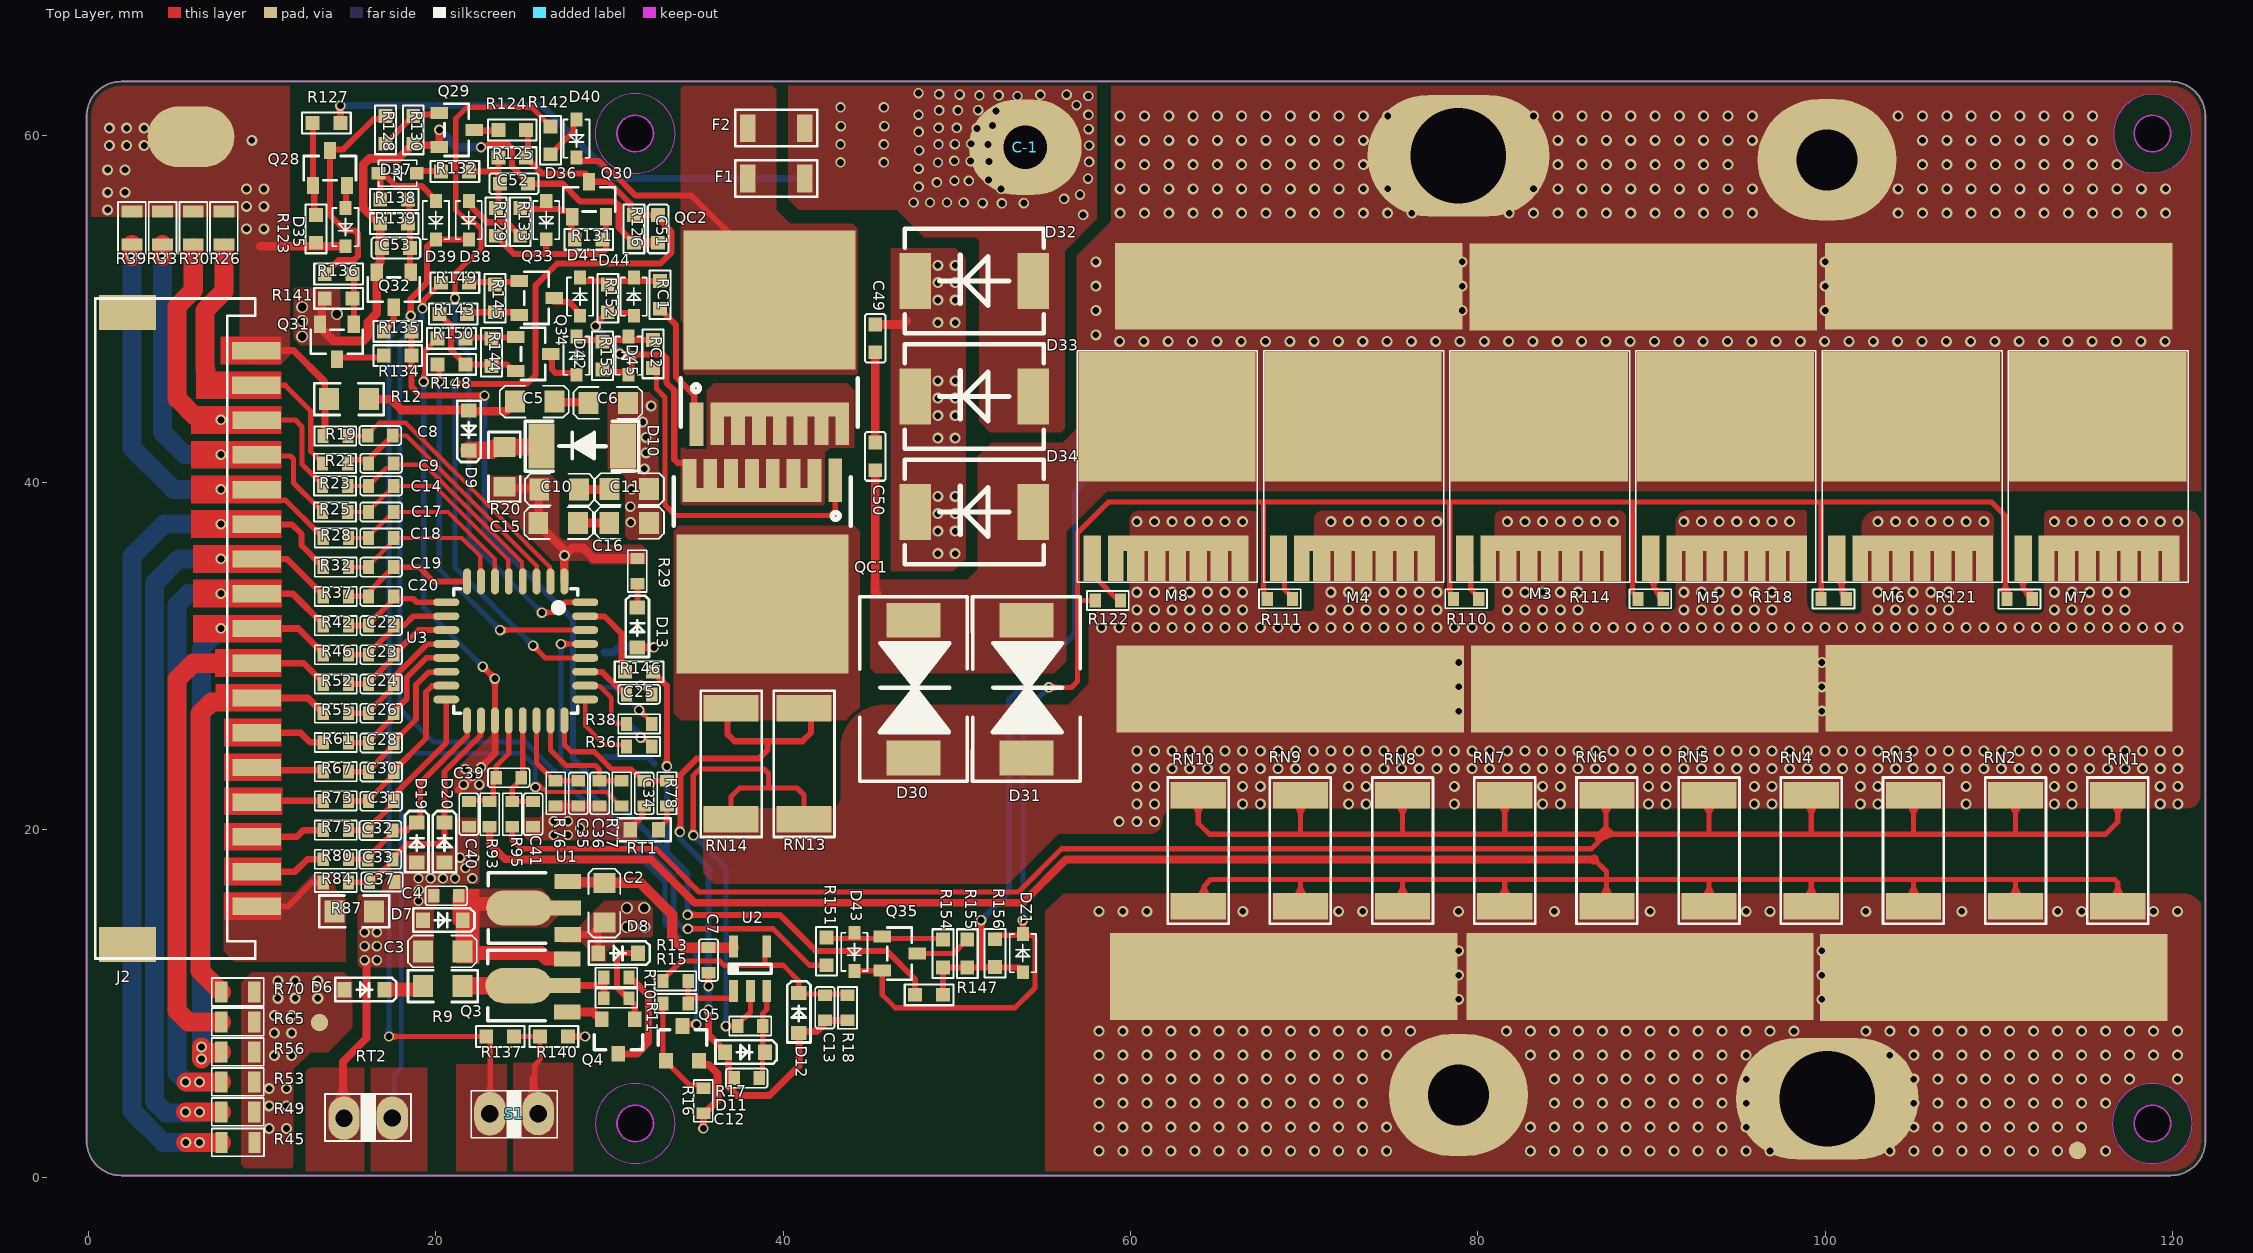
[diagram p0: Top Layer view]
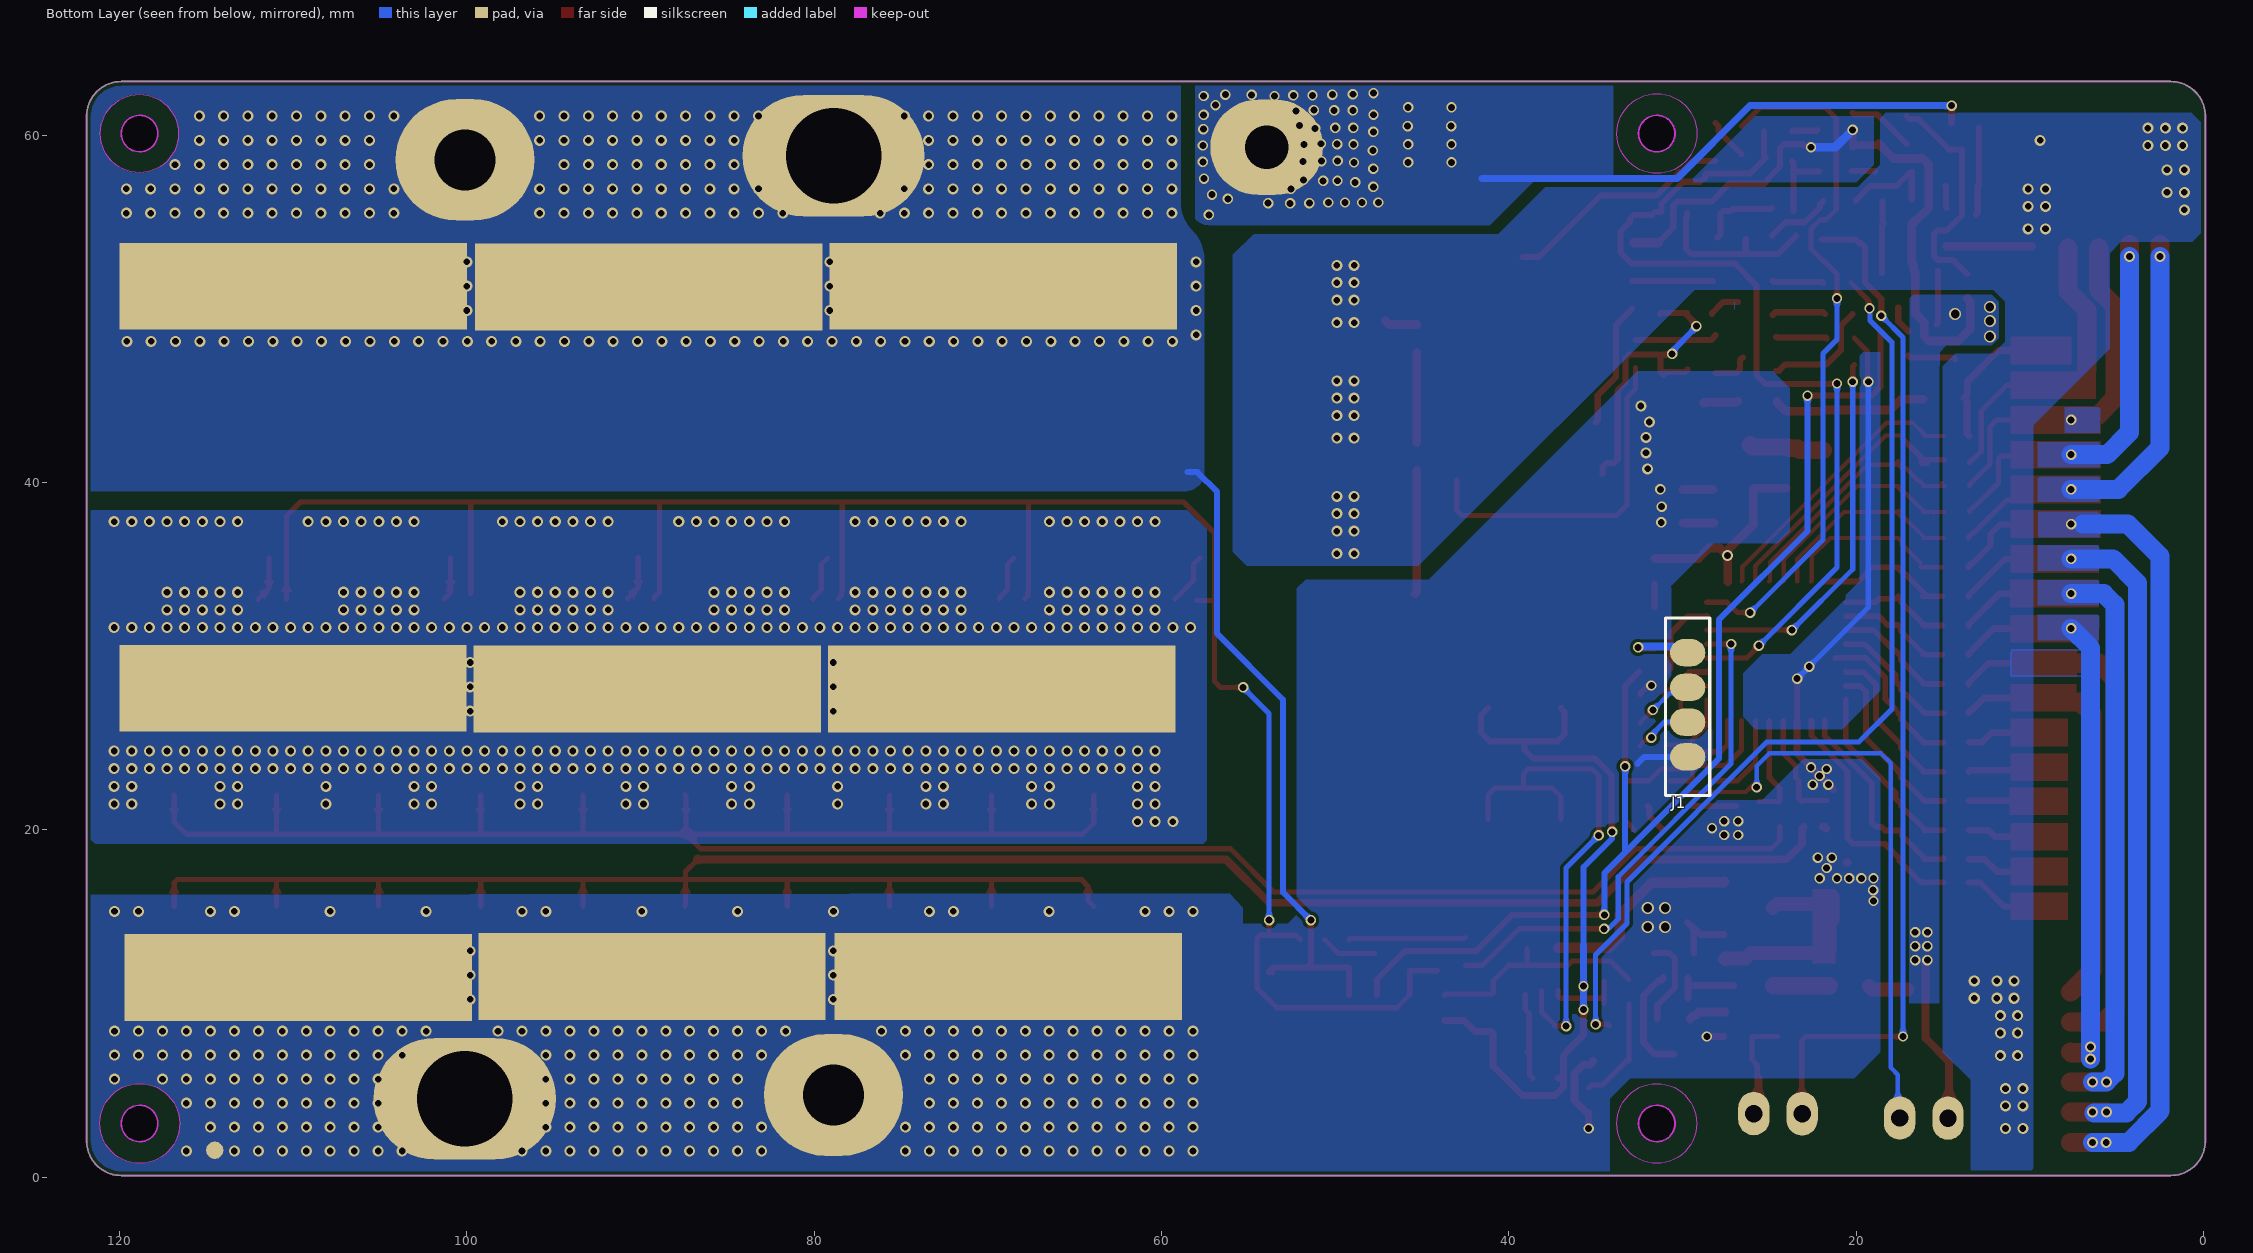
[diagram p1: Bottom Layer view, seen from below]
# Altium PCB MISC86327.PcbDoc (part 1 of 2)
Units mm, origin at the board's own origin, x right, y up, seen from the top; angles counter-clockwise.
Board outline 122 x 63 mm, 2 copper layers (Top Layer, Bottom Layer); 198 components, 117 nets, 551 pads, 998 vias.
Unrouted connection lines stored in the file: 65.

## Layer stack, top to bottom (the 12.6 mil dielectric is the usual default, probably not edited)
Top Solder: solder mask 0.0102, Solder Resist, Dk 3.5
Top Layer: signal copper 0.0356
Dielectric 1: dielectric 0.32, FR-4, Dk 4.8
Bottom Layer: signal copper 0.0356
Bottom Solder: solder mask 0.0102, Solder Resist, Dk 3.5

## Board outline
-0.11,2.09 -0.11,61.09 cw(c1.89,61.09) 1.89,63.09 119.89,63.09 cw(c119.89,61.09) 121.89,61.09 121.89,2.09 cw(c119.89,2.09) 119.89,0.09 1.89,0.09 cw(c1.89,2.09)
cut-out: 31.48,59.04 cw(c31.48,60.09) 30.43,60.09 cw(c31.48,60.09) 31.48,61.14 cw(c31.48,60.09) 32.53,60.09 cw(c31.48,60.09)
cut-out: 30.43,3.09 ccw(c31.48,3.09) 31.48,2.04 ccw(c31.48,3.09) 32.53,3.09 ccw(c31.48,3.09) 31.48,4.14 ccw(c31.48,3.09)
cut-out: 117.79,3.09 ccw(c118.84,3.09) 118.84,2.04 ccw(c118.84,3.09) 119.89,3.09 ccw(c118.84,3.09) 118.84,4.14 ccw(c118.84,3.09)
cut-out: 117.79,60.09 ccw(c118.84,60.09) 118.84,59.04 ccw(c118.84,60.09) 119.89,60.09 ccw(c118.84,60.09) 118.84,61.14 ccw(c118.84,60.09)

## Design rules (kind name [scope] priority, off if disabled: settings)
Clearance [All] p1: gap=0.2 ignorepadtopadclearanceinfootprint=FALSE except(0: Arc-Hole Track-Hole SMDPad-Hole THPad-Hole Via-Hole Fill-Hole Poly-Hole Region-Hole Text-Hole)
ComponentClearance [All] p1 off: gap=0.254 collisioncheckmode=3 verticalgap=0.254 showdistances=FALSE
Height [All] p1 off: minheight=0 maxheight=25.4 prefheight=12.7
HoleSize [All] p1: absolutevalues=TRUE maxlimit=10 minlimit=0.025 maxpercent=80.000 minpercent=20.000
HoleToHoleClearance [All] p1 off: gap=0 allowstackedmicrovias=TRUE
MinimumSolderMaskSliver [All] p1 off: minsoldermaskwidth=0
PolygonConnect [All] p1: connectstyle=Direct reliefconductorwidth=0.254 reliefentries=4 polygonreliefangle="90 Angle" airgapwidth=0.254
RoutingVias [All] p1: holewidth=0.5 width=0.8 viastyle="Through Hole" minholewidth=0.4 minwidth=0.6 maxholewidth=0.711 maxwidth=1.27
SilkToSilkClearance [All] p1 off: silktosilkclearance=0
SilkToSolderMaskClearance [IsPad] p1 off: minsilkscreentomaskgap=0 clearancetoexposedcopper=TRUE
SolderMaskExpansion [All] p1: expansion=0.102 istentingtop=FALSE
SupplyNets "Schematic Supply Nets_2" [InNet('DSGD1')] p1: voltage=0.000
SupplyNets "Schematic Supply Nets_5" [InNet('C-')] p2: voltage=0.000
SupplyNets "Schematic Supply Nets" [InNet('BC16')] p3: voltage=0.000
SupplyNets "Schematic Supply Nets_6" [InNet('GND1')] p4: voltage=0.000
SupplyNets "Schematic Supply Nets_4" [InNet('5V')] p5: voltage=0.000
SupplyNets "Schematic Supply Nets_3" [InNet('GND')] p6: voltage=0.000
Width [All] p1: maxlimit=20 minlimit=0.2 preferedwidth=0.3
23 further rules are at their usual default settings.

## Components (designator, comment, footprint, x,y, rotation, side; value= is the part's Value field where it differs from the comment)
C2 "10uF/25V" C0805 29.7,15.8 r270 top
C3 "2.2uF/50V" C0805 20.4,13 r180 top
C4 "0.1uF" C0603M 20.6,16.2 r180 top
C5 "2.2uF/100V" C0805 25.69,44.66 r180 top
C6 "2.2uF/100V" C0805 29.93,44.58 r180 top
C7 "10nF" C0603M 35.7,12.5 r270 top
C8 "0.1uF" C0603M 16.8,42.7 r0 top
C9 "0.1uF" C0603M 16.845,41.1 r0 top
C10 "0.1uF/100V" C0805 27.095,39.582 r0 top
C11 "0.1uF/100V" C0805 31.135,39.612 r0 top
C12 "0.47uF" C0603M 37.9,5.7 r180 top
C13 "0.47uF" C0603M 42.4,9.753 r270 top
C14 "0.1uF" C0603M 16.847,39.8 r0 top
C15 "2.2uF/100V" C0805 27.039,37.662 r0 top
C16 "2.2uF/100V" C0805 31.125,37.672 r0 top
C17 "0.1uF" C0603M 16.847,38.3 r0 top
C18 "0.1uF" C0603M 16.847,36.806 r0 top
C19 "0.1uF" C0603M 16.847,35.123 r0 top
C20 "0.1uF" C0603M 16.847,33.441 r0 top
C22 "0.1uF" C0603M 16.847,31.759 r0 top
C23 "0.1uF" C0603M 16.847,30.077 r0 top
C24 "0.1uF" C0603M 16.847,28.395 r0 top
C25 "1uF/25V" C0603M 31.7,27.8 r0 top
C26 "0.1uF" C0603M 16.847,26.713 r0 top
C28 "0.1uF" C0603M 16.847,25 r0 top
C30 "0.1uF" C0603M 16.847,23.33 r0 top
C31 "0.1uF" C0603M 16.847,21.648 r0 top
C32 "0.1uF" C0603M 16.8,19.966 r0 top
C33 "0.1uF" C0603M 16.8,18.3 r0 top
C34 "102" C0603M 32,22.1 r90 top
C35 "102" C0603M 28.2,22.1 r90 top
C36 "102" C0603M 29.43,22.1 r90 top
C37 "1uF" C0603M 16.9,17 r0 top
C39 "102" C0603M 24.2,23 r180 top
C40 "1uF" C0603M 21.9,20.9 r270 top
C41 "1uF" C0603M 25.6,20.9 r270 top
C49 "0.1uF" C0603A 45.3,48.3 r90 top
C50 "0.1uF" C0603A 45.3,41.5 r90 top
C51 "0.1uF" C0603A 32.8,54.6 r90 top
C52 "0.1uF" C0603A 24.5,57.2 r180 top
C53 "0.1uF" C0603A 17.7,53.5 r0 top
C-1 "Pth" 4*3 53.94,59.3 r0 top locked
D6 "1N4148WS" SOD-323-E 15.9,10.8 r0 top
D7 "15V" SOD-323-E 20.4,14.8 r0 top
D8 "15V" SOD-323-E 30.5,12.9 r0 top
D9 "BAV21WS" SOD-323-E 21.9,43 r270 top
D10 "SMAJ64A" SMA 28.43,42.09 r180 top
D11 "1N4148WS" SOD-323-E 37.8,7.2 r0 top
D12 "1N4148WS" SOD-323-E 40.9,9.453 r90 top
D13 "BAV21WS" SOD-323-E 31.6,31.65 r90 top
D19 "BAT46WS" SOD-323-E 18.9,19.261 r90 top
D20 "BAT46WS" SOD-323-E 20.5,19.261 r90 top
D30 "SMDJ150CA" SMC-BI 47.5,28.1 r90 top
D31 "SMDJ150CA" SMC-BI 54,28.1 r90 top
D32 "RS5M" SMC_MDO-214AB) 51,51.6 r180 top
D33 "RS5M" SMC_MDO-214AB) 51,44.95 r180 top
D34 "RS5M" SMC_MDO-214AB) 51,38.3 r180 top
D35 "15V" SOD323(A+K-) 14.8,54.7 r90 top
D36 "5.6V" SOD323(A+K-) 26.357,55.106 r90 top
D37 "1N4148WS" SOD323(A+K-) 17.8,57.8 r0 top
D38 "1N4148WS" SOD323(A+K-) 21.9,55.1 r90 top
D39 "1N4148WS" SOD323(A+K-) 20,55.1 r90 top
D40 "BAV21WS" SOD323(A+K-) 28.1,59.8 r90 top
D41 "1N4148WS" SOD323(A+K-) 28.3,50.7 r270 top
D42 "BAV21WS" SOD323(A+K-) 28.1,47.3 r270 top
D43 "BAV21WS" SOD323(A+K-) 44.1,12.975 r90 top
D44 "15V" SOD323(A+K-) 31.4,50.7 r270 top
D45 "15V" SOD323(A+K-) 31.1,47.3 r270 top
DZ1 "15V" SOD323(A+K-) 53.8,12.9 r270 top
F1 "5A/125VAC" R1206L 39.6,57.5 r0 top
F2 "40A/72V" R1206L 39.6,60.4 r0 top
J1 "UART_M" CON4/2.0 29.7,27.2 r270 bottom
J2 "PH-2.0mm-17P right-angle connector without latch" "HY2.0WT-17A/P 卧贴带扣耐温260℃" 5.965,31.59 r90 top locked
M3 "SP012N02AGHTO" TOLL#1 83.487,39.712 r0 top
M4 "SP012N02AGHTO" TOLL#1 72.768,39.712 r0 top
M5 "SP012N02AGHTO" TOLL#1 94.205,39.712 r0 top
M6 "SP012N02AGHTO" TOLL#1 104.923,39.712 r0 top
M7 "SP012N02AGHTO" TOLL#1 115.642,39.712 r0 top
M8 "SP012N02AGHTO" TOLL#1 62.05,39.712 r0 top
Q3 "DXT5551" SOT-89BCE 26.159,11.028 r90 top
Q4 "MMBT5551" SOT-23S 30.5,8.1 r180 top
Q5 "MMBT5551" SOT-23S 34.2,7.7 r0 top
Q28 "MMBT5401" SOT23-3_BEC 13.9,58.1 r0 top
Q29 "MMBT5551" SOT23-3_BEC 21.2,60.3 r270 top
Q30 "MMBT5401" SOT23-3_BEC 28.825,56.3 r0 top
Q31 "MMBT5551" SOT23-3_BEC 14.3,48.1 r180 top
Q32 "MMBT5551" SOT23-3_BEC 17.575,51.1 r180 top
Q33 "MMBT5401" SOT23-3_BEC 25.8,50.625 r270 top
Q34 "MMBT5401" SOT23-3_BEC 25.6,47.4 r270 top
Q35 "MMBT5401" SOT23-3_BEC 46.7,12.875 r270 top
QC1 "N MOS*" TOLL#2 38.8,36.5 r180 top
QC2 "N MOS*" TOLL#2 39.2,47 r0 top
R9 "200R" R0805 20.4,11 r180 top
R10 "100K" R0603m 30.4,11.5 r0 top
R11 "3M" R0603m 30.4,10.3 r0 top
R12 "1K" R0805 15,44.8 r0 top
R13 "470K 1%" R0603m 33.8,11.3 r0 top
R15 "100K 1%" R0603m 33.8,10 r180 top
R16 "1M" R0603m 35.4,4.4 r90 top
R17 "1K 1%" R0603m 38.1,8.7 r180 top
R18 "1K 1%" R0603m 43.7,9.753 r90 top
R19 "510R" R0603m 14.222,42.675 r0 top
R20 "100R" R0805 23.942,40.895 r90 top
R21 "510R" R0603m 14.2,41.1 r0 top
R23 "510R" R0603m 14.2,39.8 r0 top
R25 "510R" R0603m 14.2,38.3 r0 top
R26 "0R/NC/17 used in series" R0805A 7.8,54.65 r270 top
R28 "510R" R0603m 14.239,36.806 r0 top
R29 "100R" R0603m 31.6,34.9 r90 top
R30 "0R/NC/16 used in series" R0805A 6.033,54.65 r270 top
R32 "510R" R0603m 14.239,35.123 r0 top
R33 "0R/NC/17 used in series" R0805A 4.267,54.65 r270 top
R36 "100R" R0603m 31.7,24.8 r180 top
R37 "510R" R0603m 14.239,33.441 r0 top
R38 "100R" R0603m 31.7,26.1 r180 top
R39 "0R/NC/16 used in series" R0805A 2.5,54.65 r270 top
R42 "510R" R0603m 14.239,31.759 r0 top
R45 "0R/NC/17 used in series" R0805A 8.6,2 r180 top
R46 "510R" R0603m 14.239,30.077 r0 top
R49 "0R/NC/16 used in series" R0805A 8.597,3.76 r180 top
R52 "510R" R0603m 14.239,28.395 r0 top
R53 "0R/NC/17 used in series" R0805A 8.597,5.485 r180 top
R55 "510R" R0603m 14.239,26.713 r0 top
R56 "0R/NC/16 used in series" R0805A 8.597,7.21 r180 top
R61 "510R" R0603m 14.239,25.03 r0 top
R65 "0R/NC/17 used in series" R0805A 8.597,8.935 r180 top
R67 "510R" R0603m 14.239,23.348 r0 top
R70 "0R/NC/16 used in series" R0805A 8.597,10.66 r180 top
R73 "510R" R0603m 14.239,21.666 r0 top
R75 "510R" R0603m 14.239,19.984 r0 top
R76 "10K" R0603m 26.9,22.1 r270 top
R77 "10R" R0603m 30.7,22.1 r270 top
R78 "1.25K 1%" R0603m 33.3,22.1 r270 top
R80 "510R" R0603m 14.239,18.302 r0 top
R84 "510R" R0603m 14.239,16.97 r0 top
R87 "51R" R0805 15.3,15.3 r180 top
R93 "10R" R0603m 23.1,20.9 r90 top
R95 "10R" R0603m 24.4,20.9 r90 top
R110 "100R" R0603m 79.325,33.3 r0 top
R111 "100R" R0603m 68.6,33.3 r0 top
R114 "100R" R0603m 89.94,33.3 r0 top
R118 "100R" R0603m 100.48,33.29 r0 top
R121 "100R" R0603m 111.19,33.28 r0 top
R122 "100R" R0603m 58.7,33.2 r0 top
R123 "20K" R0603A 13.1,54.6 r270 top
R124 "1K" R0603A 24.4,60.3 r0 top
R125 "NC" R0603A 24.4,58.7 r180 top
R126 "10M" R0603A 31.4,54.6 r90 top
R127 "100K" R0603A 13.7,60.7 r180 top
R128 "510K" R0603A 17.1,60.3 r90 top
R129 "200K" R0603A 23.457,55.006 r90 top
R130 "100K" R0603A 18.7,60.3 r90 top
R131 "150K" R0603A 28.8,54 r0 top
R132 "470K" R0603A 21.1,57.9 r180 top
R133 "680K" R0603A 24.857,55.006 r270 top
R134 "1K" R0603A 17.8,47.3 r0 top
R135 "1K" R0603A 17.8,48.7 r0 top
R136 "510K" R0603A 14.4,52 r180 top
R137 "0Ω/NC" R0603A 23.7,8.1 r0 top
R138 "150K" R0603A 17.6,56.3 r180 top
R139 "200K" R0603A 17.6,54.9 r0 top
R140 "10K" R0603A 26.8,8.1 r0 top
R141 "100K" R0603A 14.4,50.6 r0 top
R142 "3M" R0603A 26.6,59.7 r90 top
R143 "10K" R0603A 21,49.7 r180 top
R144 "1M" R0603A 23.2,47.5 r270 top
R145 "1M" R0603A 23.4,50.6 r270 top
R146 "100K" R0603A 31.7,29.1 r180 top
R147 "1M" R0603A 48.4,10.5 r180 top
R148 "1K" R0603A 20.9,46.8 r180 top
R149 "3M" R0603A 21.1,51.5 r0 top
R150 "3M" R0603A 20.9,48.3 r180 top
R151 "1K" R0603A 42.5,13 r270 top
R152 "1M" R0603A 29.9,50.6 r270 top
R153 "1M" R0603A 29.6,47.3 r90 top
R154 "4.7M" R0603A 49.2,12.875 r90 top
R155 "1K" R0603A 50.6,12.875 r270 top
R156 "10M" R0603A 52.2,12.9 r90 top
RC1 "100R" R0603A 32.9,50.8 r270 top
RC2 "100R" R0603A 32.5,47.4 r90 top
RN1 "2mR" R2512A 116.847,18.802 r90 top
RN2 "2mR" R2512A 110.964,18.802 r90 top
RN3 "2mR" R2512A 105.081,18.802 r90 top
RN4 "2mR" R2512A 99.198,18.802 r90 top
RN5 "2mR" R2512A 93.315,18.802 r90 top
RN6 "2mR" R2512A 87.432,18.802 r90 top
RN7 "2mR" R2512A 81.549,18.802 r90 top
RN8 "2mR" R2512A 75.666,18.802 r90 top
RN9 "2mR" R2512A 69.783,18.802 r90 top
RN10 "2mR" R2512A 63.9,18.802 r90 top
RN13 "10mR" R2512A 41.2,23.8 r270 top
RN14 "2mR" R2512A 37,23.8 r270 top
RT1 "10K" R0603 32,20 r180 top
RT2 "10K 3435" NTC-DIP 16.102,3.402 r180 top locked
S1 "SW-SPST" NTC-DIP 24.5,3.654 r0 top
U1 "ME6239A50PG" SO-89 26.2,15.5 r90 top
U2 "TP2121-TR" SOT23-5 38.1,12 r0 top
U3 "SH3676014B" LQFP-32 24.6,30.3 r180 top

## Footprints (in the part's own frame and the unit in brackets; to place one, negate y for a bottom-side part, rotate by r counter-clockwise, add the part's x,y. Pads: shape width x height; smd on the part's side, far side on the other; paste and mask are expansions set on the pad)
4*3 [mm] "通孔焊盘"
  oval 6.5x5.5 hole 2.5 mask+0: 1(0,0)
C0603A [mm] "贴片电容"
  rect 0.8x0.8 smd mask+0.08: 1(-0.8,0) 2(0.8,0)
  silkscreen extent -1.4,-0.6 1.4,0.6
C0603M [mm] "贴片电容"
  rect 0.65x0.8 smd mask+0.05: 1(-0.725,0) 2(0.725,0)
  silkscreen extent -1.2,-0.55 1.2,0.55
C0805 [mil]
  rect 45x50 smd: 1(-45,0) 2(45,0)
  silkscreen extent -77,-36 79,36, body extent -39,-24 39,24, height 47
CON4/2.0 [mil]
  oval 62x80 smd: 1(-118.11,0) 2(-39.37,0) 3(39.37,0) 4(118.11,0)
  silkscreen extent -197,-50 206,50
"HY2.0WT-17A/P 卧贴带扣耐温260℃" [mm] "卧贴连接器"
  rect 2x3.3 smd: 0(-18.2,3.725) 0(18.2,3.725)
  rect 1x2.8 smd: 1(-16,-3.725) 2(-14,-3.725) 3(-12,-3.725) 4(-10,-3.725) 5(-8,-3.725) 6(-6,-3.725) 7(-4,-3.725) 8(-2,-3.725) 9(0,-3.725) 10(2,-3.725) 11(4,-3.725) 12(6,-3.725) 13(8,-3.725) 14(10,-3.725) 15(12,-3.725) 16(14,-3.7) 17(16,-3.7)
  silkscreen extent -19,-3.63 19,5.57
LQFP-32 [mm]
  oval 0.45x1.5 smd mask+0.152: 1(-2.8,-4) 2(-2,-4) 3(-1.2,-4) 4(-0.4,-4) 5(0.4,-4) 6(1.2,-4) 7(2,-4) 8(2.8,-4) 17(2.8,4) 18(2,4) 19(1.2,4) 20(0.4,4) 21(-0.4,4) 22(-1.2,4) 23(-2,4) 24(-2.8,4)
  oval 1.5x0.45 smd mask+0.152: 9(4,-2.8) 10(4,-2) 11(4,-1.2) 12(4,-0.4) 13(4,0.4) 14(4,1.2) 15(4,2) 16(4,2.8) 25(-4,2.8) 26(-4,2) 27(-4,1.2) 28(-4,0.4) 29(-4,-0.4) 30(-4,-1.2) 31(-4,-2) 32(-4,-2.8)
  silkscreen extent -3.58,-3.58 3.58,3.58
NTC-DIP [mm]
  oval 1.8x2.5 hole 1: 1(-1.39,-0.005) 2(1.39,0.005)
  silkscreen extent -2.46,-1.39 2.49,1.32
R0603 [mil]
  rect 30x35 smd: 1(-32,0) 2(32,0)
  silkscreen extent -60,-26 60,26, body extent -31,-16 32,16, height 18
R0603A [mm] "贴片电阻"
  rect 0.8x0.8 smd mask+0.08: 1(-0.8,0) 2(0.8,0)
  silkscreen extent -1.4,-0.6 1.4,0.6
R0603m [mm] "贴片电阻"
  rect 0.65x0.8 smd mask+0.05: 1(-0.725,0) 2(0.725,0)
  silkscreen extent -1.21,-0.55 1.2,0.55
R0805 [mil]
  rect 45x50 smd: 1(-45,0) 2(45,0)
  silkscreen extent -79,-36 79,36
R0805A [mm] "贴片电阻"
  rect 0.7x1.2 smd paste+0 mask+0.08: 1(-0.95,0) 2(0.95,0)
  silkscreen extent -1.5,-0.8 1.5,0.8
R1206L [mm] "贴片电阻"
  rect 0.9x1.6 smd: 1(-1.65,0) 2(1.65,0)
  silkscreen extent -2.35,-1.05 2.35,1.05
R2512A [mm]
  rect 1.524x3.175 smd: 1(-3.2,0) 2(3.2,0)
  silkscreen extent -4.22,-1.75 4.21,1.76, body extent -3.06,-1.59 3.24,1.61, height 0.64
SMA [mm]
  rect 1.5x2.6 smd paste+0 mask+0: A(-2.35,0) K(2.35,0)
  silkscreen extent -3.24,-1.43 3.27,1.46, body extent -2.3,-1.35 2.3,1.35, height 2.4
SMC-BI [mm]
  rect 2x3.1 smd: A(-3.97,0) K(3.97,0)
  silkscreen extent -5.32,-3.1 5.33,3.1
SMC_MDO-214AB) [mm] "贴片二极管"
  rect 1.8x3.2 smd: 1(-3.4,0) 2(3.4,0)
  silkscreen extent -4,-3 4,3
SO-89 [mil]
  rect 34x60 smd: 1(-60,-55) 3(60,-55)
  oval 80x150 smd: 2(0,55)
  rect 34x100 smd: 2(0,-35)
  silkscreen extent -80,-5 80,125
SOD323(A+K-) [mm] "贴片二极管"
  rect 0.8x0.7 smd: A(1.1,0) K(-1.1,0)
  silkscreen extent -1.1,-0.75 1.1,0.75
SOD-323-E [mm]
  rect 0.8x0.9 smd: A(-1.15,0) K(1.15,0)
  silkscreen extent -1.7,-0.68 1.82,0.68, body extent -1.3,-0.65 1.3,0.65, height 1
SOT23-3_BEC [mm] "贴片IC/MOS*"
  rect 0.7x1 smd: B(-0.975,-1) C(0,1.016) E(0.975,-1)
  silkscreen extent -1.5,-0.7 1.5,0.7
SOT23-5 [mil]
  rect 20x50 smd: 1(-37.5,-50) 2(0.5,-50) 3(37.5,-50) 4(37.5,50) 5(-37.5,50)
  silkscreen extent -48,-10 48,10
SOT-23S [mm]
  rect 0.8x0.9 smd: B(-0.95,-1) C(0,1) E(0.95,-1)
  silkscreen extent -1.41,-0.11 1.39,0.78, body extent -1.45,-1.4 1.45,1.4, height 1.2
SOT-89BCE [mil]
  rect 34x60 smd: B(-60,-55) E(60,-55)
  oval 80x150 smd: C(0,55)
  rect 34x100 smd: C(0,-35)
  silkscreen extent -80,-5 80,125
TOLL#1 [mm]
  rect 10.2x7.45 smd: D(0.05,4.075)
  rect 1x2.61 smd: G(-4.25,-4.075) S(-1.75,-4.075) S(-0.55,-4.075) S(0.65,-4.075) S(1.85,-4.075) S(3.05,-4.075) S(4.25,-4.075)
  rect 0.9x2.61 smd: S(-2.9,-4.075)
  rect 7x0.9 smd: S(0.812,-3.22)
  silkscreen extent -5.11,-5.47 5.26,7.87
TOLL#2 [mm] "贴片MOS"
  rect 0.8x2.5 smd: 1(-4.2,-3.638)
  rect 0.8x1.7 smd: 2(-3,-4) 2(-1.8,-4) 2(-0.6,-4) 2(0.6,-4) 2(1.8,-4) 2(3,-4) 2(4.2,-4)
  rect 8x0.8 smd: 2(0.6,-2.788)
  rect 9.9x8 smd: 3(0,3.5)
  silkscreen extent -5.1,-3.8 5.1,-1

## Part data
C2 C3: library part "CAPACITOR POL", "Capacitor"
C4 C5 C6 C8 C9 C10 C11 C14 C15 C16 C17 C18 C19 C20 C22 C23 C24 C25 C26 C28 C30 C31 C32 C33 C34 C35 C36 C37 C39 C40 C41: library part CAP, "Capacitor"
C7 C12 C13: library part CAP, "CAP"
C49 C50 C51 C52 C53: library part "0805 100nF(104) 10% 50V", "chip capacitor", Package=0805, SuppliersPartNumber=C49678
C-1: "through-hole pad"
D6 D9 D11 D12 D13 D19 D20 D37 D38 D39 D40 D41 D42 D43: library part DIODE, "Diode"
D7 D8 D10 D35 D36 D44 D45 DZ1: library part ZENER2, "Zener Diode"
D30 D31: library part diode-esd, "bidirectional ESD"
D32 D33 D34: "chip diode"
F1 F2: library part FUSE1, "Fuse"
J1: library part CON4, "Connector"
J2: library part PH-2.0mm-17P弯脚不带扣
M3 M4 M5 M6 M7 M8: library part "MOSFET N"
Q3 Q4 Q5 Q29 Q31 Q32: library part NPN, "NPN Transistor"
Q28 Q30 Q33 Q34 Q35: library part PNP, "PNP Transistor"
QC1 QC2: "chip MOS"
R9 R10 R11 R12 R19 R20 R21 R23 R25 R26 R28 R29 R30 R32 R33 R36 R37 R38 R39 R42 R45 R46 R49 R52 R53 R55 R56 R61 R65 R67 R70 R73 R75 R76 R77 R78 R80 R84 R87 R93 R95 R110 R111 R114 R118 R121 R122 RN1 RN2 RN3 RN4 RN5 RN6 RN7 RN8 RN9 RN10 RN13 RN14: library part RES1
R13 R15 R16 R17 R18 R123 R124 R125 R126 R127 R128 R129 R130 R131 R132 R133 R134 R135 R136 R137 R138 R139 R140 R141 R142 R144 R146 R147 R148 R150 R151 R153 R154 R155 R156: library part RES1, "RES"
R143 R145 R149 R152: library part RES
RC1 RC2: library part "0603 1.2MΩ (1204) 1%", "chip resistor", Package=0603, SuppliersPartNumber=C22766
RT1 RT2: library part RES3
S1: "Single-Pole, Single-Throw Switch"
U1: library part VOLTREG
U2: "S8211D"
U3: library part SH3676016B

## Free pads (board coordinates)
  round 1 smd: 28(13.3,8.9) 28(114.522,1.542)
  round 1 smd far side: 29(114.51,1.55)
  oval 8x7 hole 3.5: 30(78.88,4.73) 30(100.11,58.57)
  oval 10.5x7 hole 5.5: 30(78.88,58.81) 30(100.11,4.51)
  rect 20x5 smd far side: 31(68.82,11.55) 31(69.1,51.3) 31(69.2,28.1) 31(89.33,11.55) 31(89.53,51.25) 31(89.6,28.1) 31(109.7,11.5) 31(110,51.3) 31(110.01,28.15)
  rect 20x5 smd: 32(68.82,11.55) 32(69.1,51.3) 32(69.2,28.1) 32(89.33,11.55) 32(89.53,51.25) 32(89.6,28.1) 32(109.7,11.5) 32(110,51.3) 32(110.01,28.15)
  oval 5x3.5 smd: B(5.9,59.9)

## Via types
v1: diameter 0.635, hole 0.381, Top Layer to Bottom Layer, tented both sides, 846 vias
v2: diameter 0.6, hole 0.4, Top Layer to Bottom Layer, tented both sides, 133 vias
v3: diameter 0.635, hole 0.4, Top Layer to Bottom Layer, tented both sides, 11 vias
v4: diameter 0.7, hole 0.5, Top Layer to Bottom Layer, tented both sides, 8 vias

## Nets (pads, with @x,y where several pads share a name; then routed paths per layer and width w, separated by ;. In a path a pad name is that pad's centre, name@x,y a point inside that pad or via, vN(x,y) a via of type N, cw(c..) or ccw(c..) an arc to the next point about the centre after c; other vN are vias at no path point)
5V: C2.1 C7.1 U1.3 U2.5 | length 11.9
  Top Layer w0.6: U1.3@27.597,17.024 27.638,16.984 29.66,16.984 C2.1@29.7,16.943 31.759,16.943 33.6,15.102 33.6,13.8 34.2,13.2 U2.5@37.148,13.2
BC0: J2.1 R84.1 R87.2 | length 4.4
  Top Layer w0.35: J2.1@9.69,15.59 11.49,15.59 12.869,16.969 R84.1@13.514,16.97 R84.1@13.514,16.97
BC1: J2.2 R80.1 | length 4.1
  Top Layer w0.381: J2.2@9.69,17.59 11.89,17.59 12.602,18.302 R80.1@13.514,18.302
BC2: J2.3 R75.1 | length 4
  Top Layer w0.381: J2.3@9.69,19.59 11.99,19.59 12.384,19.984 R75.1@13.514,19.984
BC3: J2.4 R73.1 | length 3.9
  Top Layer w0.381: J2.4@9.69,21.59 9.766,21.666 R73.1@13.514,21.666
BC4: J2.5 R67.1 | length 4.5
  Top Layer w0.381: J2.5@9.125,23.6 9.302,23.423 13.439,23.423 R67.1@13.514,23.348
BC5: J2.6 R61.1 | length 4.1
  Top Layer w0.381: J2.6@9.69,25.59 12.21,25.59 12.77,25.03 R61.1@13.514,25.03
BC6: J2.7 R55.1 R70.2 | length 23.9
  Top Layer w0.381: J2.7@9.69,27.59 12.637,27.59 13.304,26.922 13.379,26.922 13.514,26.788 R55.1@13.514,26.713
  Top Layer w1.1: R70.2@7.647,10.66 6.434,11.873 6.434,26.706 7.079,27.35 8.973,27.35 J2.7@9.223,27.6
BC7: J2.8 R52.1 R65.2 | length 31.2
  Top Layer w0.381: J2.8@9.69,29.59 12.394,29.59 13.514,28.47 R52.1@13.514,28.395
  Top Layer w1.1: R65.2@7.647,8.935 5.744,8.935 5.1,9.579 5.1,28.666 6.024,29.59 J2.8@9.69,29.59
BC8: J2.9 R46.1 R56.2 | length 31.3
  Top Layer w0.381: J2.9@9.69,31.59 12.076,31.59 13.514,30.152 R46.1@13.514,30.077
  Top Layer w1.1: v3(6.5,6.8) v3(6.5,7.5) ; 6.86,7.16 7.597,7.16 R56.2@7.647,7.21
  Bottom Layer w1.1: v3(6.5,6.8) v3(6.5,7.5) 6.5,30.475 v2(7.625,31.6)
BC9: J2.10 R42.1 R53.2 | length 37.9
  Top Layer w0.381: J2.10@9.69,33.59 9.7,33.6 11.748,33.6 13.514,31.834 R42.1@13.514,31.759
  Top Layer w0.75: R53.2@7.647,5.485 R53.2@7.657,5.475
  Top Layer w1.1: v3@5.607,5.475 R53.2@7.657,5.475
  Bottom Layer w1.1: v3(6.379,5.485) v3(5.597,5.485) 5.1,5.982 5.1,32.956 5.744,33.6 v2(7.625,33.6)
BC10: J2.11 R37.1 R49.2 | length 43.8
  Top Layer w0.35: J2.11@9.69,35.59 11.44,35.59 13.514,33.516 R37.1@13.514,33.441
  Top Layer w1.1: v3(5.597,3.76) v3(6.379,3.76) R49.2@7.647,3.76
  Bottom Layer w1.1: v3@6.3,3.7 4.444,3.7 3.8,4.344 3.8,34.2 5.2,35.6 v2(7.625,35.6)
BC11: J2.12 R32.1 R45.2 | length 49.1
  Top Layer w0.35: J2.12@9.69,37.59 11.71,37.59 12.269,37.031 12.269,36.369 13.289,35.348 13.364,35.348 13.514,35.198 R32.1@13.514,35.123
  Top Layer w1.1: v3(5.6,2) v3(6.382,2) R45.2@7.65,2
  Bottom Layer w1.1: v3(6.382,2) 4.306,2 2.5,3.806 2.5,35.756 4.344,37.6 6.925,37.6
  other v2: 7.625,37.6
BC12: J2.13 R28.1 R39.2 | length 22.8
  Top Layer w0.3: J2.13@9.69,39.59 10.301,38.979 11.341,38.979 13.264,37.056 13.339,37.056 13.514,36.881 R28.1@13.514,36.806
  Top Layer w1.1: v3(2.5,53) R39.2@2.5,53.7
  Bottom Layer w1.1: v3(2.5,53) 2.5,42 4.9,39.6 v2(7.625,39.6)
BC13: J2.14 R25.1 R33.2 | length 20.7
  Top Layer w0.3: J2.14@9.69,41.59 9.749,41.531 11.624,41.531 11.8,41.355 11.8,39.975 13.225,38.55 13.3,38.55 13.475,38.375 R25.1@13.475,38.3
  Top Layer w1.1: v3(4.267,53) R33.2@4.267,53.7
  Bottom Layer w1.1: v3(4.267,53) 4.267,42.878 5.544,41.6 v2(7.625,41.6)
BC14: J2.15 R23.1 R30.2 | length 18.7
  Top Layer w0.3: J2.15@9.69,43.59 11.91,43.59 12.3,43.2 12.3,41.05 13.475,39.875 R23.1@13.475,39.8
  Top Layer w1.1: R30.2@6.033,53.5 6.033,51.072 5.1,50.138 5.1,44.839 6.089,43.85 7.375,43.85 v2(7.625,43.6)
BC15: J2.16 R21.1 R26.2 | length 17.2
  Top Layer w0.3: J2.16@9.665,45.59 9.675,45.6 11.322,45.6 12.8,44.122 12.8,41.795 13.245,41.35 13.3,41.35 13.475,41.175 R21.1@13.475,41.12
  Top Layer w1.1: R26.2@7.8,53.5 7.8,51 6.7,49.9 6.7,46.494 6.75,46.444 6.75,45.85 7,45.6 J2.16@8.65,45.6
BC16: C49.2 D6.A D32.2 D33.2 D34.2 D35.K J2.17 pad.28@13.3,8.9 pad.B R12.1 R19.1 R26.1 R30.1 R33.1 R39.1 R45.1 R49.1 R53.1 R56.1 R65.1 R70.1 R123.2 | length 15.4
  Top Layer w0.4: J2.17@9.1,47.6 J2.17@9.665,47.6 ; J2.17@9.665,47.59 11.81,47.59 13.601,45.799 13.601,45.056 13.799,44.858 13.622,44.681 13.622,42.8 R19.1@13.497,42.675
  Top Layer w0.5: 9.9,53.6 D35.K@14.8,53.6 ; C49.2@45.3,49.1 46.9,49.1 47.1,49.3
  other v1: 10.4,2.8 11.4,2.8 10.4,4.1 11.4,4.1 10.4,5.1 11.4,5.1 10.7,7 11.7,7 10.7,8.3 11.7,8.3 10.7,9.3 11.7,9.3 10.9,10.3 11.9,10.3 13.2,10.3 10.9,11.3 11.9,11.3 13.2,11.3 48.9,35.9 49.9,35.9 48.9,37.2 49.9,37.2 48.9,38.2 49.9,38.2 48.9,39.2 49.9,39.2 48.9,42.55 49.9,42.55 48.9,43.85 49.9,43.85 48.9,44.85 49.9,44.85 48.9,45.85 49.9,45.85 48.9,49.2 49.9,49.2 48.9,50.5 49.9,50.5 48.9,51.5 49.9,51.5 48.9,52.5 49.9,52.5 9.1,54.6 10.1,54.6 1.1,55.7 9.1,55.9 10.1,55.9 1.1,56.7 2.1,56.7 9.1,56.9 10.1,56.9 1.1,58 2.1,58 1.2,59.4 2.2,59.4 3.2,59.4 9.4,59.7 1.2,60.4 2.2,60.4 3.2,60.4
C-: C-1.1 D32.1 D33.1 F1.2 F2.2 R127.1 | length 29.8
  Top Layer w0.4: R127.1@14.5,60.7 v2(14.5,61.7)
  Bottom Layer w0.4: v2(14.5,61.7) 26.1,61.7 30.3,57.5 41.538,57.5
  other v2: 57.272,55.412 51.482,56.082 52.592,56.072 53.862,56.082 47.512,56.122 48.452,56.122 49.432,56.122 50.392,56.122 56.18,56.33 57.092,56.572 52.552,56.902 47.802,57.022 48.852,57.282 50.692,57.362 49.862,57.372 51.822,57.422 57.552,57.492 47.802,58.062 43.3,58.43 45.8,58.43 48.912,58.422 57.612,58.462 50.792,58.502 51.842,58.482 49.852,58.512 47.822,59.112 57.612,59.402 43.3,59.47 45.8,59.47 51.802,59.462 48.942,59.472 49.882,59.482 50.812,59.502 47.802,60.192 57.582,60.342 51.152,60.392 48.952,60.422 49.992,60.412 43.32,60.52 45.82,60.52 52.042,60.552 47.792,61.172 57.57,61.17 52.252,61.392 48.982,61.422 50.062,61.422 51.222,61.442 43.3,61.6 45.8,61.6 56.89,61.73 53.492,62.252 57.572,62.252 51.302,62.292 52.402,62.292 54.812,62.312 50.162,62.332 56.322,62.332 48.982,62.352 47.792,62.422
CHG1: Q34.E R143.2 R144.2 R148.1 | length 6.6
  Top Layer w0.35: R143.2@20.2,49.7 20.875,49.025 20.875,47.625 R148.1@21.7,46.8 23.2,46.8 24.075,46.8 24.45,46.425 Q34.E@24.6,46.425
CHGD1: D40.K F1.1 F2.1 QC2.3 | length 13.4
  Top Layer w0.35: D40.K@28.1,58.5 29.4,58.5 30.034,57.866 30.17,57.866 31.517,56.519 34.719,56.519 38.25,52.988 QC2.3@39.2,52.988
CO2: Q5.C R149.1 | length 54.7
  Top Layer w0.3: v2(19.229,50.029) 19.287,50.087 19.287,50.487 R149.1@20.3,51.5 ; Q5.C@34.2,8.7 34.3,8.8 v2(35,8.8)
  Bottom Layer w0.3: v2(19.229,50.029) 19.204,50.004 19.204,49.331 17.941,48.067 17.941,26.959 19.85,25.05 25.15,25.05 33.2,17 33.2,14.6 35,12.8 v2(35,8.8)
CTLD: C51.2 Q30.C R124.2 R125.1 R126.2 U3.28 | length 52
  Top Layer w0.3: v2(25.6,30.6) 26.3,29.9 U3.28@28.6,29.9
  Top Layer w0.35: v2(21.1,45.7) 21.125,45.675 25.23,45.675 25.741,46.186 25.741,51.366 26.975,52.6 32.93,52.6 33.575,53.245 33.575,54.425 33.025,54.975 33.025,55.175 C51.2@32.8,55.4 31.763,55.4 31.581,55.581 31.219,55.581 31.208,55.592 31.208,56.05 29.942,57.316 29,57.316 Q30.C@28.9,57.416 ; R125.1@25.2,58.7 26.1,57.8 28.6,57.8 28.7,57.7 Q30.C@28.7,57.516 ; R125.1@25.3,58.7 R124.2@25.3,60.2
  Bottom Layer w0.3: v2(21.1,45.7) 21.1,35.1 v2(25.6,30.6)
DG-: D30.A D31.A M3.S M4.S M5.S M6.S M7.S M8.S pad.31@69.2,28.1 pad.31@89.6,28.1 pad.31@110.01,28.15 pad.32@69.2,28.1 pad.32@89.6,28.1 pad.32@110.01,28.15 R17.2 R95.1 RN1.2 RN2.2 RN3.2 RN4.2 RN5.2 RN6.2 RN7.2 RN8.2 RN9.2 RN10.2 RN13.2 RN14.2 U2.2 | length 172.2
  Top Layer w0.3: R95.1@24.4,20.175 24.4,19.4 24.89,18.91 32.67,18.91 35.155,16.425 53.541,16.425 56.026,18.91 86.54,18.91 87.37,19.74 ; v2(34.825,19.676) 34.825,23.125 35.2,23.5 38.9,23.5 39.15,23.25 39.15,22.4 ; v2(36.7,8.7) R17.2@37.375,8.7 37.375,8.775 38.113,9.513 U2.2@38.113,10.73 ; RN14.2@37,20.6 37,21.9 37.5,22.4 39.15,22.4 ; RN13.2@41.2,20.6 41.2,22 40.8,22.4 39.15,22.4 ; RN10.2@63.9,22.002 63.9,20.38 64.54,19.74 69.8,19.74 ; RN9.2@69.783,22.002 69.783,19.757 69.8,19.74 ; RN8.2@75.666,22.002 75.666,19.744 75.67,19.74 ; RN7.2@81.549,22.002 81.549,19.769 81.52,19.74 ; RN6.2@87.432,22.002 87.37,21.94 87.37,19.74 ; RN5.2@93.315,22.002 93.315,19.745 93.32,19.74 ; RN4.2@99.198,22.002 99.198,19.778 99.16,19.74 ; RN3.2@105.081,22.002 105.081,19.809 105.15,19.74 ; RN2.2@110.964,22.002 110.964,19.844 110.86,19.74 ; RN1.2@116.847,22.002 116.847,20.447 116.14,19.74 110.86,19.74 ; 69.8,19.74 75.67,19.74 ; 75.67,19.74 81.52,19.74 ; 81.52,19.74 87.37,19.74 ; 87.37,19.74 93.32,19.74 ; 93.32,19.74 99.16,19.74 ; 99.16,19.74 105.15,19.74 ; 105.15,19.74 110.86,19.74
  Bottom Layer w0.3: v2@34.8,19.701 36.7,17.801 v2(36.7,8.7)
  other v1: 59.346,20.47 60.362,20.47 61.378,20.47 60.362,21.486 61.378,21.486 66.458,21.486 67.474,21.486 72.554,21.486 73.57,21.486 78.65,21.486 83.73,21.486 84.746,21.486 89.826,21.486 90.842,21.486 95.922,21.486 96.938,21.486 102.018,21.486 103.034,21.486 108.114,21.486 113.194,21.486 114.21,21.486 119.29,21.486 120.306,21.486 60.362,22.502 61.378,22.502 66.458,22.502 67.474,22.502 72.554,22.502 73.57,22.502 78.65,22.502 83.73,22.502 84.746,22.502 89.826,22.502 90.842,22.502 95.922,22.502 96.938,22.502 102.018,22.502 103.034,22.502 108.114,22.502 113.194,22.502 114.21,22.502 119.29,22.502 120.306,22.502 60.362,23.518 61.378,23.518 62.394,23.518 63.41,23.518 64.426,23.518 65.442,23.518 66.458,23.518 67.474,23.518 68.49,23.518 69.506,23.518 70.522,23.518 71.538,23.518 72.554,23.518 73.57,23.518 74.586,23.518 75.602,23.518 76.618,23.518 77.634,23.518 78.65,23.518 79.666,23.518 80.682,23.518 81.698,23.518 82.714,23.518 83.73,23.518 84.746,23.518 85.762,23.518 86.778,23.518 87.794,23.518 88.81,23.518 89.826,23.518 90.842,23.518 91.858,23.518 92.874,23.518 93.89,23.518 94.906,23.518 95.922,23.518 96.938,23.518 97.954,23.518 98.97,23.518 99.986,23.518 101.002,23.518 102.018,23.518 103.034,23.518 104.05,23.518 105.066,23.518 106.082,23.518 107.098,23.518 108.114,23.518 109.13,23.518 110.146,23.518 111.162,23.518 112.178,23.518 113.194,23.518 114.21,23.518 115.226,23.518 116.242,23.518 117.258,23.518 118.274,23.518 119.29,23.518 120.306,23.518 60.362,24.534 61.378,24.534 62.394,24.534 63.41,24.534 64.426,24.534 65.442,24.534 66.458,24.534 67.474,24.534 68.49,24.534 69.506,24.534 70.522,24.534 71.538,24.534 72.554,24.534 73.57,24.534 74.586,24.534 75.602,24.534 76.618,24.534 77.634,24.534 78.65,24.534 79.666,24.534 80.682,24.534 81.698,24.534 82.714,24.534 83.73,24.534 84.746,24.534 85.762,24.534 86.778,24.534 87.794,24.534 88.81,24.534 89.826,24.534 90.842,24.534 91.858,24.534 92.874,24.534 93.89,24.534 94.906,24.534 95.922,24.534 96.938,24.534 97.954,24.534 98.97,24.534 99.986,24.534 101.002,24.534 102.018,24.534 103.034,24.534 104.05,24.534 105.066,24.534 106.082,24.534 107.098,24.534 108.114,24.534 109.13,24.534 110.146,24.534 111.162,24.534 112.178,24.534 113.194,24.534 114.21,24.534 115.226,24.534 116.242,24.534 117.258,24.534 118.274,24.534 119.29,24.534 120.306,24.534 99.802,26.832 78.89,26.833 78.89,28.233 99.802,28.232 78.89,29.633 99.802,29.632 58.33,31.646 59.346,31.646 60.362,31.646 61.378,31.646 62.394,31.646 63.41,31.646 64.426,31.646 65.442,31.646 66.458,31.646 67.474,31.646 68.49,31.646 69.506,31.646 70.522,31.646 71.538,31.646 72.554,31.646 73.57,31.646 74.586,31.646 75.602,31.646 76.618,31.646 77.634,31.646 78.65,31.646 79.666,31.646 80.682,31.646 81.698,31.646 82.714,31.646 83.73,31.646 84.746,31.646 85.762,31.646 86.778,31.646 87.794,31.646 88.81,31.646 89.826,31.646 90.842,31.646 91.858,31.646 92.874,31.646 93.89,31.646 94.906,31.646 95.922,31.646 96.938,31.646 97.954,31.646 98.97,31.646 99.986,31.646 101.002,31.646 102.018,31.646 103.034,31.646 104.05,31.646 105.066,31.646 106.082,31.646 107.098,31.646 108.114,31.646 109.13,31.646 110.146,31.646 111.162,31.646 112.178,31.646 113.194,31.646 114.21,31.646 115.226,31.646 116.242,31.646 117.258,31.646 118.274,31.646 119.29,31.646 120.306,31.646 60.362,32.662 61.378,32.662 62.394,32.662 63.41,32.662 64.426,32.662 65.442,32.662 66.458,32.662 71.538,32.662 72.554,32.662 73.57,32.662 74.586,32.662 75.602,32.662 76.618,32.662 77.634,32.662 81.698,32.662 82.714,32.662 83.73,32.662 84.746,32.662 85.762,32.662 91.858,32.662 92.874,32.662 93.89,32.662 94.906,32.662 95.922,32.662 96.938,32.662 103.034,32.662 104.05,32.662 105.066,32.662 106.082,32.662 107.098,32.662 113.194,32.662 114.21,32.662 115.226,32.662 116.242,32.662 117.258,32.662 60.362,33.678 61.378,33.678 62.394,33.678 63.41,33.678 64.426,33.678 65.442,33.678 66.458,33.678 71.538,33.678 72.554,33.678 73.57,33.678 74.586,33.678 75.602,33.678 76.618,33.678 77.634,33.678 81.698,33.678 82.714,33.678 83.73,33.678 84.746,33.678 85.762,33.678 91.858,33.678 92.874,33.678 93.89,33.678 94.906,33.678 95.922,33.678 96.938,33.678 103.034,33.678 104.05,33.678 105.066,33.678 106.082,33.678 107.098,33.678 113.194,33.678 114.21,33.678 115.226,33.678 116.242,33.678 117.258,33.678 60.362,37.742 61.378,37.742 62.394,37.742 63.41,37.742 64.426,37.742 65.442,37.742 66.458,37.742 71.538,37.742 72.554,37.742 73.57,37.742 74.586,37.742 75.602,37.742 76.618,37.742 77.634,37.742 81.698,37.742 82.714,37.742 83.73,37.742 84.746,37.742 85.762,37.742 86.778,37.742 87.794,37.742 91.858,37.742 92.874,37.742 93.89,37.742 94.906,37.742 95.922,37.742 96.938,37.742 97.954,37.742 103.034,37.742 104.05,37.742 105.066,37.742 106.082,37.742 107.098,37.742 108.114,37.742 109.13,37.742 113.194,37.742 114.21,37.742 115.226,37.742 116.242,37.742 117.258,37.742 118.274,37.742 119.29,37.742 120.306,37.742
DSG1: D43.A Q35.B R151.1 R154.2 | length 6.8
  Top Layer w0.3: R151.1@42.5,13.8 42.562,13.738 49.137,13.738 R154.2@49.2,13.675
DSGD: R134.2 R135.2 R146.1 R147.2 | length 68.6
  Top Layer w0.35: R135.2@18.6,48.7 R134.2@18.6,47.3 18.6,45.5 19.1,45 v2(22.8,45) ; R146.1@32.5,29.1 33.3,28.3 v2(33.3,23.65) ; v2(34.5,15.1) 39.8,15.1 41.875,13.025 45.955,13.025 47.6,11.38 R147.2@47.6,10.5
  Bottom Layer w0.35: v2(22.8,45) 22.8,37.2 27.9,32.1 27.9,24.1 33.3,18.7 ; v2(33.3,23.65) 33.3,18.7 ; v2(34.5,15.1) 34.5,17.5 33.3,18.7
DSGD1: C50.1 D30.K D31.K D34.1 DZ1.A M3.D M4.D M5.D M6.D M7.D M8.D pad.30@78.88,58.81 pad.30@100.11,58.57 pad.31@69.1,51.3 pad.31@89.53,51.25 pad.31@110,51.3 pad.32@69.1,51.3 pad.32@89.53,51.25 pad.32@110,51.3 R147.1 R154.1 R155.2 R156.1 | length 45.4
  Top Layer w0.35: R147.1@49.2,10.5 R154.1@49.2,12.075 R155.2@50.6,12.075 51.6,12.075 ; v2(51.4,14.8) 51.4,12.275 51.6,12.075 ; DZ1.A@53.6,11.775 DZ1.A@53.6,11.8 ; DZ1.A@53.8,11.8 53.8,11.85 53.575,12.075 51.6,12.075
  Top Layer w0.5: C50.1@45.3,40.7 45.3,33.7 45.4,33.6
  Bottom Layer w0.35: v2(51.4,14.8) 53,16.4 53,27.5 56.8,31.3 56.8,39.46 57.94,40.6 58.5,40.6
  other v1: 59.37,48.12 60.77,48.12 62.17,48.12 63.57,48.12 64.97,48.12 66.37,48.12 67.77,48.12 69.17,48.12 70.57,48.12 71.97,48.12 73.37,48.12 74.77,48.12 76.17,48.12 77.57,48.12 78.97,48.12 80.37,48.12 81.77,48.12 83.17,48.12 84.57,48.12 85.97,48.12 87.37,48.12 88.77,48.12 90.17,48.12 91.57,48.12 92.97,48.12 94.37,48.12 95.77,48.12 97.17,48.12 98.57,48.12 99.97,48.12 101.37,48.12 102.77,48.12 104.17,48.12 105.57,48.12 106.97,48.12 108.37,48.12 109.77,48.12 111.17,48.12 112.57,48.12 113.97,48.12 115.37,48.12 116.77,48.12 118.17,48.12 119.57,48.12 58.002,48.502 58.002,49.902 79.09,49.903 100.002,49.902 58.002,51.302 79.09,51.303 100.002,51.302 58.002,52.702 79.09,52.703 100.002,52.702 59.402,55.502 60.802,55.502 62.202,55.502 63.602,55.502 65.002,55.502 66.402,55.502 67.802,55.502 69.202,55.502 70.602,55.502 72.002,55.502 73.402,55.502 74.802,55.502 76.202,55.502 81.802,55.502 83.202,55.502 84.602,55.502 86.002,55.502 87.402,55.502 88.802,55.502 90.202,55.502 91.602,55.502 93.002,55.502 94.402,55.502 95.802,55.502 104.202,55.502 105.602,55.502 107.002,55.502 108.402,55.502 109.802,55.502 111.202,55.502 112.602,55.502 114.002,55.502 115.402,55.502 116.802,55.502 118.202,55.502 119.602,55.502 59.402,56.902 60.802,56.902 62.202,56.902 63.602,56.902 65.002,56.902 66.402,56.902 67.802,56.902 69.202,56.902 70.602,56.902 72.002,56.902 73.402,56.902 74.802,56.902 83.202,56.902 84.602,56.902 86.002,56.902 87.402,56.902 88.802,56.902 90.202,56.902 91.602,56.902 93.002,56.902 94.402,56.902 95.802,56.902 104.202,56.902 105.602,56.902 107.002,56.902 108.402,56.902 109.802,56.902 111.202,56.902 112.602,56.902 114.002,56.902 115.402,56.902 116.802,56.902 118.202,56.902 119.602,56.902 59.402,58.302 60.802,58.302 62.202,58.302 63.602,58.302 65.002,58.302 66.402,58.302 67.802,58.302 69.202,58.302 70.602,58.302 72.002,58.302 73.402,58.302 84.602,58.302 86.002,58.302 87.402,58.302 88.802,58.302 90.202,58.302 91.602,58.302 93.002,58.302 94.402,58.302 105.602,58.302 107.002,58.302 108.402,58.302 109.802,58.302 111.202,58.302 112.602,58.302 114.002,58.302 115.402,58.302 116.802,58.302 59.402,59.702 60.802,59.702 62.202,59.702 63.602,59.702 65.002,59.702 66.402,59.702 67.802,59.702 69.202,59.702 70.602,59.702 72.002,59.702 73.402,59.702 84.602,59.702 86.002,59.702 87.402,59.702 88.802,59.702 90.202,59.702 91.602,59.702 93.002,59.702 94.402,59.702 95.802,59.702 105.602,59.702 107.002,59.702 108.402,59.702 109.802,59.702 111.202,59.702 112.602,59.702 114.002,59.702 115.402,59.702 59.402,61.102 60.802,61.102 62.202,61.102 63.602,61.102 65.002,61.102 66.402,61.102 67.802,61.102 69.202,61.102 70.602,61.102 72.002,61.102 73.402,61.102 74.802,61.102 83.202,61.102 84.602,61.102 86.002,61.102 87.402,61.102 88.802,61.102 90.202,61.102 91.602,61.102 93.002,61.102 94.402,61.102 95.802,61.102 104.202,61.102 105.602,61.102 107.002,61.102 108.402,61.102 109.802,61.102 111.202,61.102 112.602,61.102 114.002,61.102 115.402,61.102